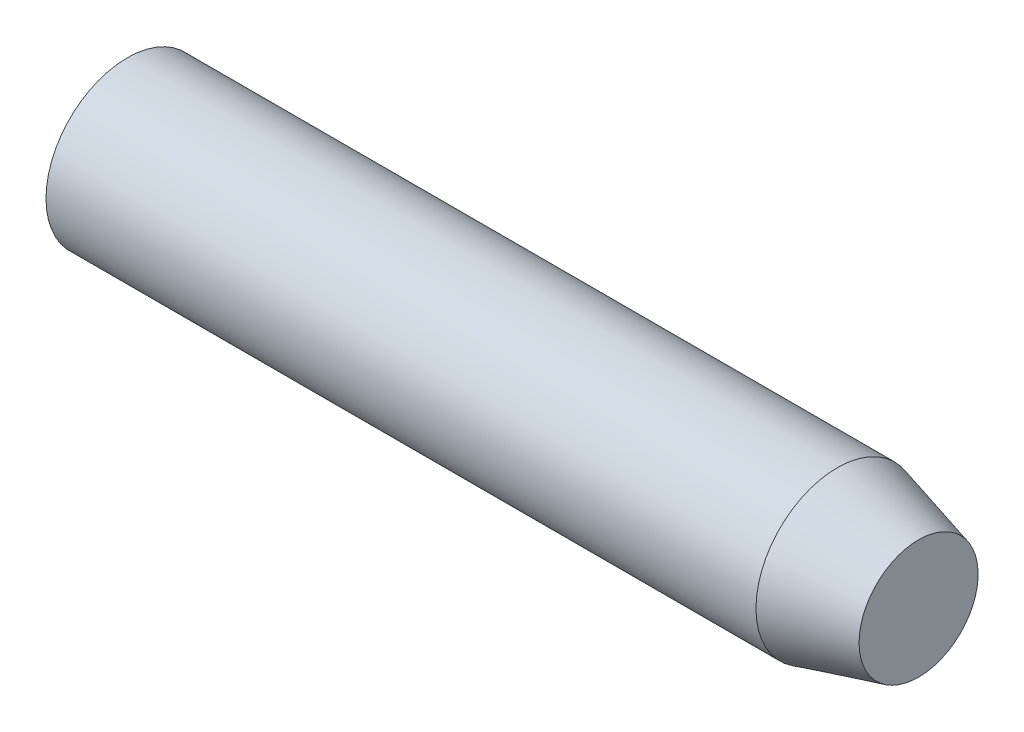
from build123d import *


with BuildPart() as part:
    # Sketch1 → Revolve1 (revolve)
    with BuildSketch(Plane(origin=(0, 0, 0), x_dir=(1, 0, 0), z_dir=(0, 1, 0))):
        with BuildLine():
            Line((-1, -1), (0, -0.732050808))
            Line((0, -0.732050808), (0, 0))
            Line((0, 0), (-10, 0))
            ThreePointArc((-10, 0), (-9.931851653, -0.51763809), (-9.732050808, -1))
            Line((-9.732050808, -1), (-1, -1))
        make_face()
    revolve(axis=Axis((-11.390713055, 0, 0), (1, 0, 0)))


solid = part.part
